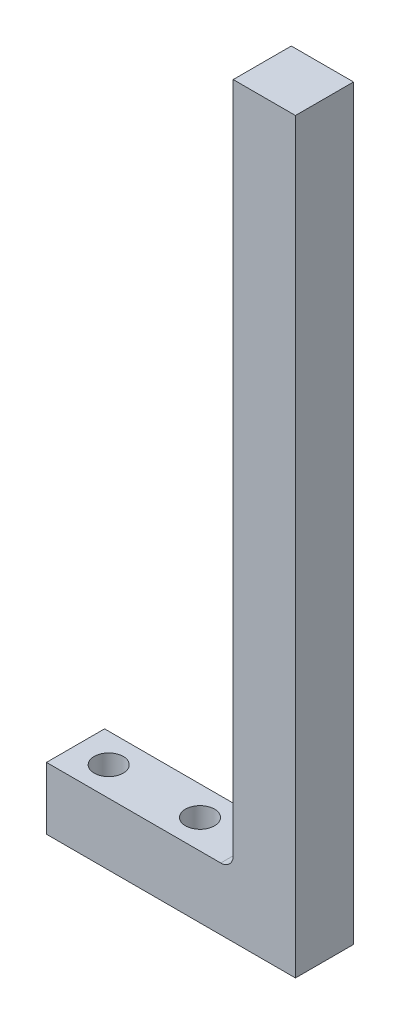
from build123d import *

# Parameters (mm, degrees)
EXTRUDE_1_DEPTH     = 7
FILLET_1_R          = 3
CUT_EXTRUDE_1_REACH = 177.71
SKETCH_3_R          = 3.5


with BuildPart() as part:
    # 草图1 → 凸台-拉伸1 (new, symmetric)
    with BuildSketch(Plane.XY):
        Polygon((0, 180), (-15, 180), (-15, 15), (-60, 15), (-60, 0), (0, 0), align=None)
    extrude(amount=EXTRUDE_1_DEPTH, both=True)

    # 圆角1
    fillet_1_edges = [part.edges().sort_by_distance(p)[0] for p in [
        (-15, 15, 0),
    ]]
    fillet(fillet_1_edges, radius=FILLET_1_R)

    # 草图3 → 切除-拉伸1 (cut, up to next)
    with BuildSketch(Plane(origin=(0, 15, 0), x_dir=(1, 0, 0), z_dir=(0, 1, 0)), mode=Mode.PRIVATE) as cut_extrude_1_sk1:
        with Locations(Location((-52, 0, 0), (0, 0, 180))):
            Circle(SKETCH_3_R)
    cut_extrude_1_tool1 = extrude(cut_extrude_1_sk1.sketch, amount=-CUT_EXTRUDE_1_REACH, mode=Mode.PRIVATE) & part.part
    # 草图3 → 切除-拉伸1 (cut, up to next)
    with BuildSketch(Plane(origin=(0, 15, 0), x_dir=(1, 0, 0), z_dir=(0, 1, 0)), mode=Mode.PRIVATE) as cut_extrude_1_sk2:
        with Locations(Location((-30, 0, 0), (0, 0, 180))):
            Circle(SKETCH_3_R)
    cut_extrude_1_tool2 = extrude(cut_extrude_1_sk2.sketch, amount=-CUT_EXTRUDE_1_REACH, mode=Mode.PRIVATE) & part.part
    add(cut_extrude_1_tool1.solids().sort_by_distance((-52, 15, 0))[0], mode=Mode.SUBTRACT)
    add(cut_extrude_1_tool2.solids().sort_by_distance((-30, 15, 0))[0], mode=Mode.SUBTRACT)


solid = part.part
